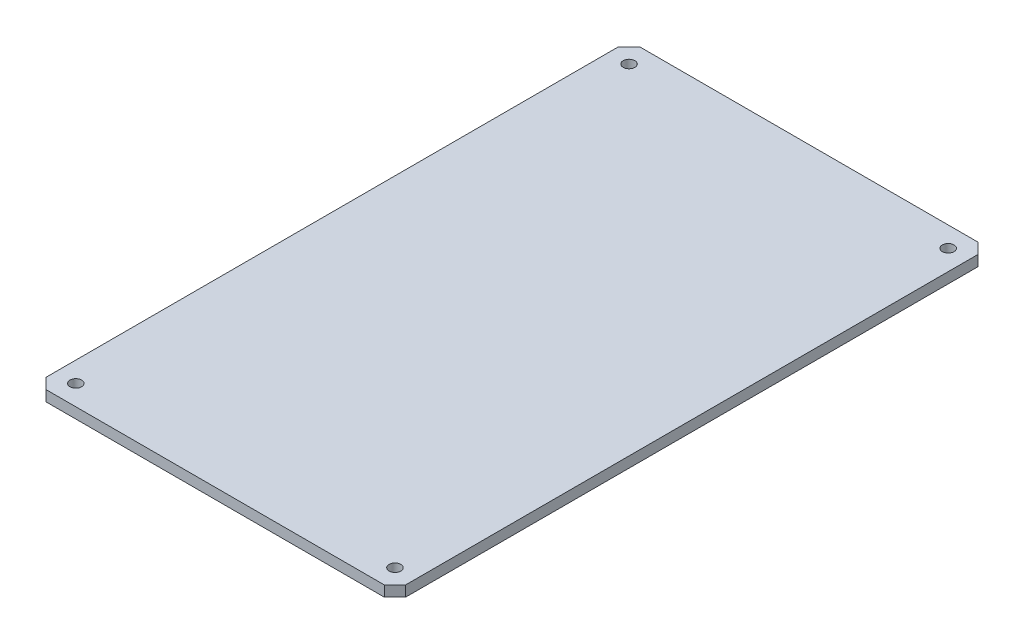
from build123d import *

# Parameters (mm, degrees)
SKETCH_1_W              = 169
SKETCH_1_H              = 279
EXTRUDE_1_DEPTH         = 2.5
HOLE_WIZARD_5_5_5_5_1_D = 5.5
CHAMFER_1_SIZE          = 5


with BuildPart() as part:
    # 草图1 → 凸台-拉伸1 (new, symmetric)
    with BuildSketch(Plane(origin=(0, 0, 0), x_dir=(1, 0, 0), z_dir=(0, 1, 0))):
        Rectangle(SKETCH_1_W, SKETCH_1_H)
    extrude(amount=EXTRUDE_1_DEPTH, both=True)

    # Ø5.5 (5.5) 直径孔1 (through all)
    with Locations(Plane(origin=(0, -2.5, 0), x_dir=(-1, 0, 0), z_dir=(0, -1, 0))):
        with Locations((75, -130), (-75, -130), (-75, 130), (75, 130)):
            Hole(HOLE_WIZARD_5_5_5_5_1_D / 2)

    # 倒角1
    chamfer_1_edges = [part.edges().sort_by_distance(p)[0] for p in [
        (-84.5, 0, -139.5),
        (84.5, 0, -139.5),
        (84.5, 0, 139.5),
        (-84.5, 0, 139.5),
    ]]
    chamfer(chamfer_1_edges, length=CHAMFER_1_SIZE)


solid = part.part
